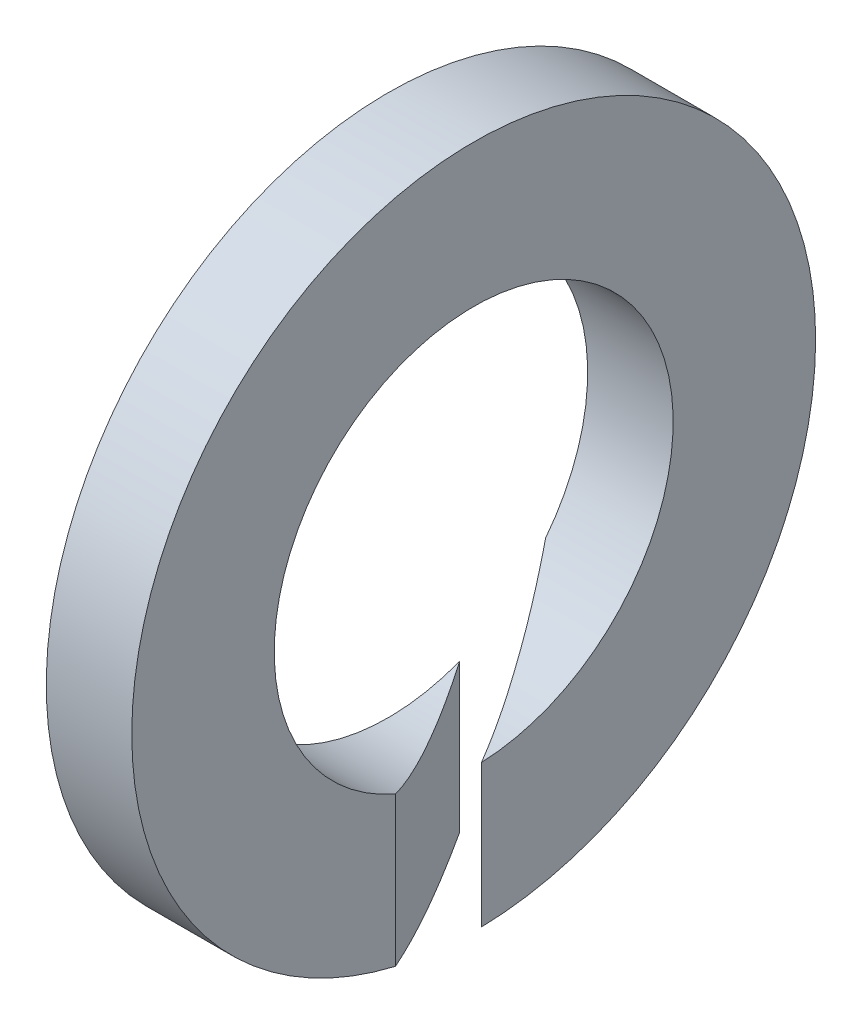
SolidWorks part; units mm, degrees
ref_plane "Front" through (0, 0, 0) normal (0, 0, 1) x (1, 0, 0)
ref_plane "Top" through (0, 0, 0) normal (0, 1, 0) x (1, 0, 0)
ref_plane "Right" through (0, 0, 0) normal (1, 0, 0) x (0, 0, -1)
sketch "Sketch1" plane through (0, 0, 0) normal (0, 0, 1) x (1, 0, 0)
  line L0 (0, 0) -> (25.3434, 0) construction
  line L1 (12.4826, 7) -> (15.4826, 7)
  line L2 (12.4826, 7) -> (12.4826, 12)
  line L3 (12.4826, 12) -> (15.4826, 12)
  line L4 (15.4826, 7) -> (15.4826, 12)
  dimension "D1" = 5
  dimension "D2" = 7
  dimension "D3" = 3
revolve "Revolve1" add sketch "Sketch1" angle 360 about L0
sketch "Sketch3" plane through (0, 0, 0) normal (0, 1, 0) x (1, 0, 0)
  line L0 (7.6947, 13.9028) -> (23.9536, -14.5502)
  line L1 (23.9536, -14.5502) -> (22.6533, -15.2932)
  line L2 (22.6533, -15.2932) -> (5.9698, 13.9028)
  line L3 (5.9698, 13.9028) -> (7.6947, 13.9028)
  dimension "D1" = 1.4977
extrude "Cut-Extrude1" cut sketch "Sketch3" against normal up to next
